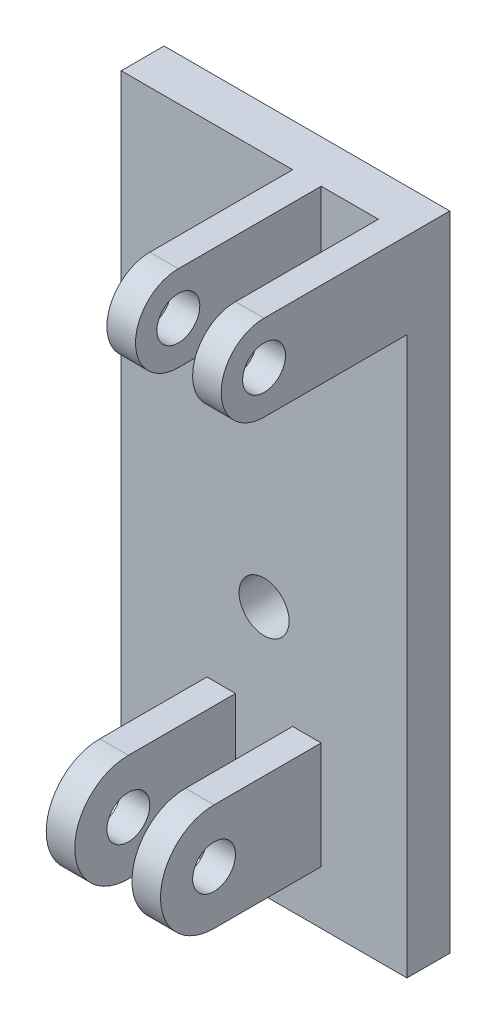
SolidWorks part; units mm, degrees
ref_plane "Front Plane" through (0, 0, 0) normal (0, 0, 1) x (1, 0, 0)
ref_plane "Top Plane" through (0, 0, 0) normal (0, 1, 0) x (1, 0, 0)
ref_plane "Right Plane" through (0, 0, 0) normal (1, 0, 0) x (0, 0, -1)
sketch "Sketch1" plane through (0, 0, 0) normal (0, 0, 1) x (1, 0, 0)
  line L1 (-20, 45) -> (20, 45)
  line L2 (-20, 45) -> (-20, -45)
  line L3 (-20, -45) -> (20, -45)
  line L4 (20, 45) -> (20, -45)
  line L5 (-20, 45) -> (20, -45) construction
  line L6 (-20, -45) -> (20, 45) construction
  point P0 (0, 0)
  dimension "D1" = 90
  dimension "D2" = 40
extrude "Boss-Extrude1" add sketch "Sketch1" along normal blind 6
sketch "Sketch3" plane through (20, 0, 0) normal (-1, 0, 0) x (0, 0, 1)
  line L0 (6, 45) -> (0, 45) construction
  line L1 (6, 45) -> (6, -45) construction
  line L2 (26, 45) -> (6, 45)
  line L3 (6, 45) -> (6, 33)
  line L4 (6, 33) -> (26, 33)
  circle A0 centre (26, 39) radius 3
  arc A1 (26, 33) -> (26, 45) centre (26, 39) ccw
  dimension "D2" = 6
  dimension "D3" = 12
  dimension "D1" = 20
extrude "Boss-Extrude2" add sketch "Sketch3" along normal blind 4
sketch "Sketch4" plane through (0, 0, 0) normal (1, 0, 0) x (0, 0, -1)
  line L0 (-6, -45) -> (-6, 33) construction
  line L1 (-21, -22.5) -> (-6, -22.5)
  line L2 (-6, -22.5) -> (-6, -37.5)
  line L3 (-6, -37.5) -> (-21, -37.5)
  circle A0 centre (-21, -30) radius 3
  arc A1 (-21, -22.5) -> (-21, -37.5) centre (-21, -30) ccw
  dimension "D1" = 6
  dimension "D2" = 15
  dimension "D3" = 15
  dimension "D4" = 30
extrude "Boss-Extrude3" add sketch "Sketch4" along normal blind 4 from offset 4
mirror "Mirror1" about plane through (0, 0, 0) normal (1, 0, 0) of "Boss-Extrude3"
pattern_linear "LPattern1" count 2 spacing 12 along (-1, 0, 0) of "Boss-Extrude2"
sketch "Sketch5" plane through (0, 0, 6) normal (0, 0, 1) x (1, 0, 0)
  circle A0 centre (0, 20) radius 3.5
  circle A1 centre (0, -10) radius 3.5
  dimension "D1" = 20
  dimension "D2" = 10
  dimension "D3" = 7
extrude "Cut-Extrude1" cut sketch "Sketch5" against normal through all
